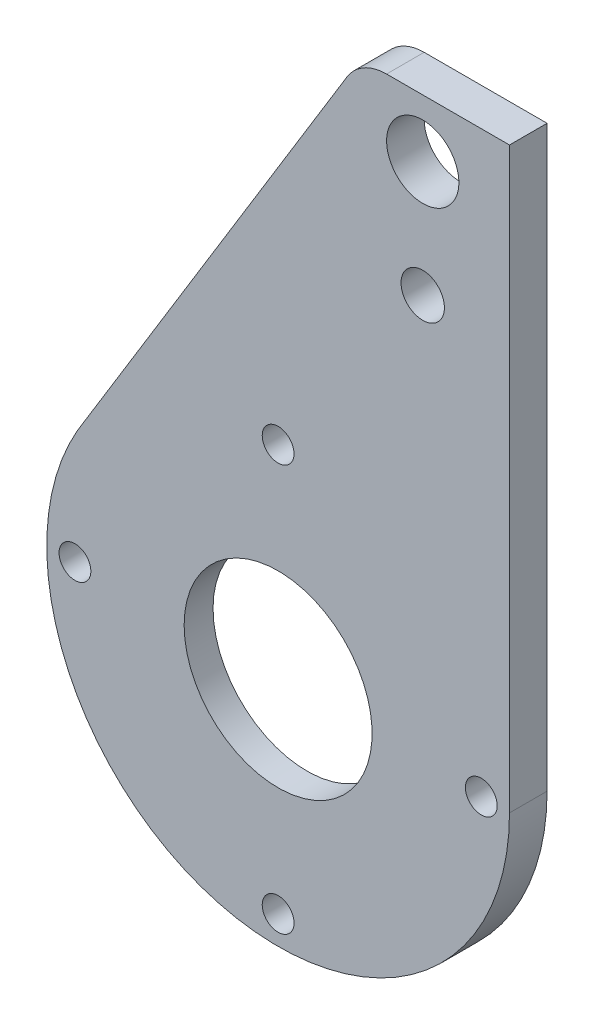
SolidWorks part; units mm, degrees
material "6061-T6 (SS)"
ref_plane "前视基准面" through (0, 0, 0) normal (0, 0, 1) x (1, 0, 0)
ref_plane "上视基准面" through (0, 0, 0) normal (0, 1, 0) x (1, 0, 0)
ref_plane "右视基准面" through (0, 0, 0) normal (1, 0, 0) x (0, 0, -1)
other "Configuration Table"
sketch "草图1" plane through (0, 0, 0) normal (0, 0, 1) x (1, 0, 0)
  line L0 (80, 200) -> (37.5, 200)
  line L1 (80, 0) -> (80, 160)
  line L4 (80, 200) -> (80, 160)
  line L7 (-69.3887, 39.8146) -> (23.8485, 192.3448)
  arc A0 (-69.3887, 39.8146) -> (80, 0) centre (0, 0) ccw
  circle A1 centre (0, 0) radius 32.5
  arc A5 (37.5, 200) -> (23.8485, 192.3448) centre (37.5, 184) ccw
  circle A6 centre (50, 180) radius 12.5
  circle A7 centre (50, 140) radius 7.5
  point P10 (34, 220)
  dimension "D1" = 160
  dimension "D2" = 65
  dimension "D5" = 40
  dimension "D4" = 25
  dimension "D3" = 15
  dimension "D7" = 16
extrude "凸台-拉伸1" add sketch "草图1" along normal blind 13
sketch "草图2" plane through (0, 0, 0) normal (0, 0, 1) x (1, 0, 0)
  circle A0 centre (0, 0) radius 60.5
  dimension "D1" = 121
extrude "切除-拉伸2" cut sketch "草图2" against normal through all from offset 3 contours A0
sketch "草图3" plane through (0, 0, 13) normal (0, 0, 1) x (1, 0, 0)
sketch "草图4" plane through (0, 0, 0) normal (0, 0, -1) x (-1, 0, 0)
  circle A0 centre (0, 0) radius 70.25 construction
  circle A1 centre (70.25, 0) radius 5.5
  circle A2 centre (0, -70.25) radius 5.5
  circle A3 centre (-70.25, 0) radius 5.5
  circle A4 centre (0, 70.25) radius 5.5
  point P14 (0, 0)
  dimension "D1" = 140.5
  dimension "D2" = 11
  dimension "D3" = 4
extrude "切除-拉伸3" cut sketch "草图4" against normal through all
